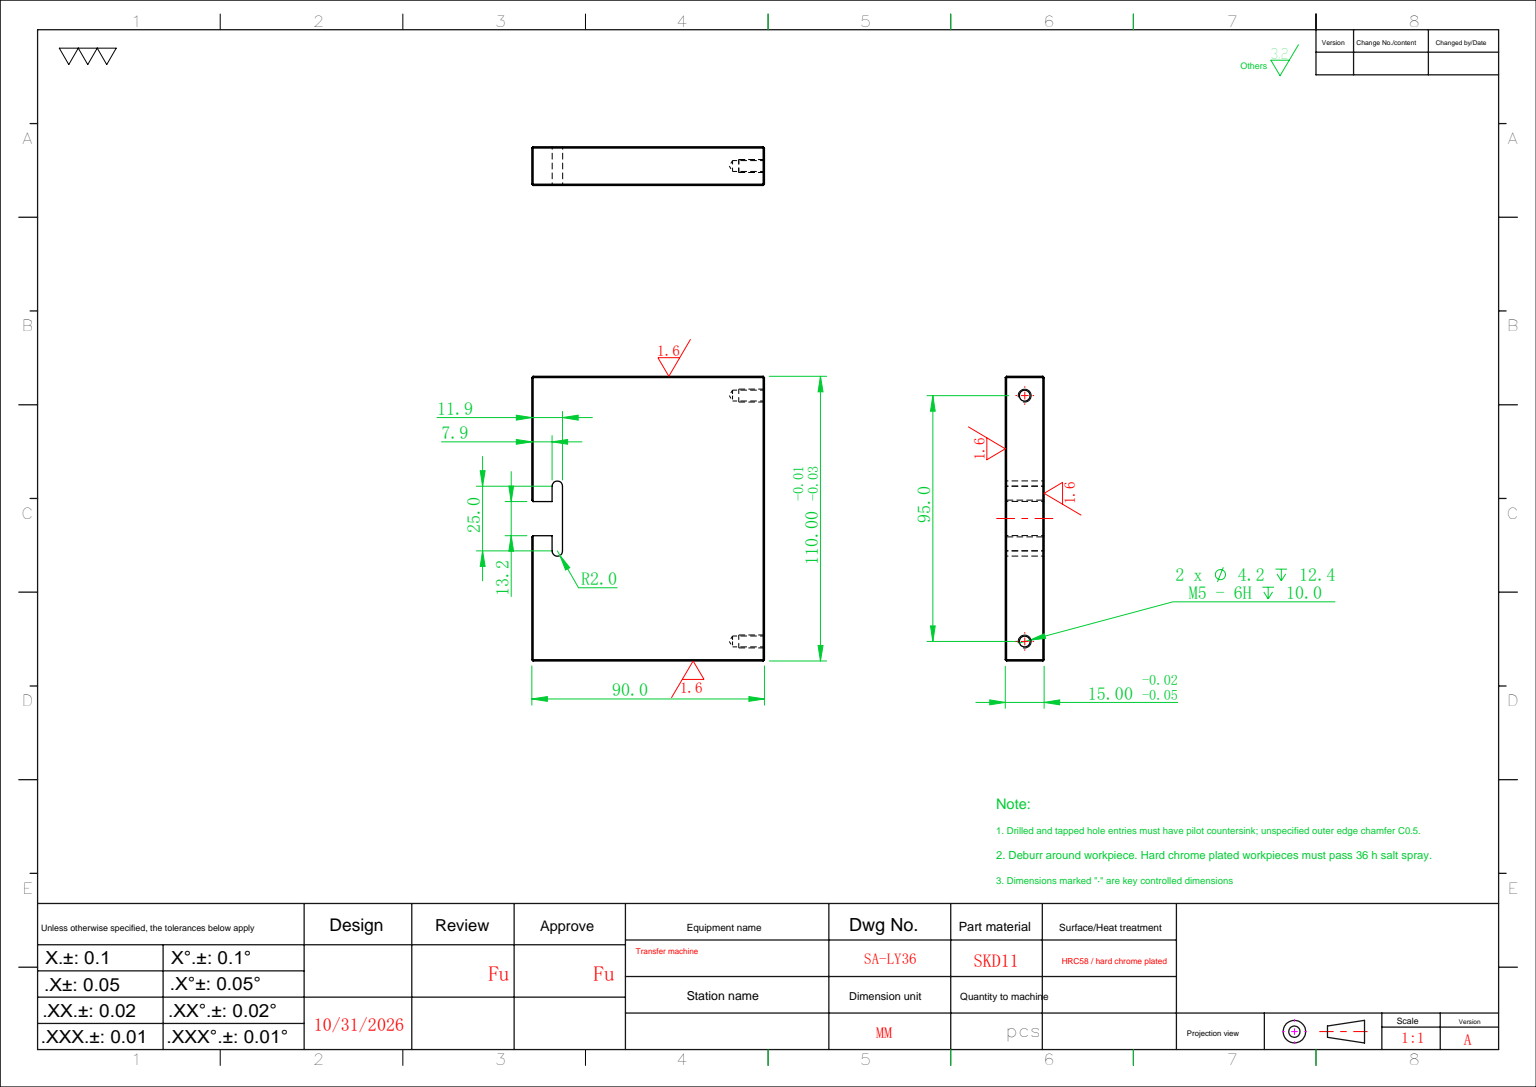
from build123d import *

# Parameters (mm, degrees)
SKETCH_1_W               = 110
SKETCH_1_H               = 90
EXTRUDE_1_DEPTH          = 15
CUT_EXTRUDE_1_DEPTH      = 73.629195232
CUT_EXTRUDE_1_DEPTH_BACK = 73.629195232
SKETCH_2_W               = 13.2
SKETCH_2_H               = 11.9
CUT_EXTRUDE_2_DEPTH      = 73.629195232
HOLE_WIZARD_M5_1_D       = 4.2
HOLE_WIZARD_M5_1_DEPTH   = 12.4
HOLE_WIZARD_M5_1_TIP     = 1.2618073
CHAMFER_1_SIZE           = 0.5


with BuildPart() as part:
    # 草图1 → 凸台-拉伸1 (new body)
    with BuildSketch(Plane.XY):
        Rectangle(SKETCH_1_W, SKETCH_1_H)
    extrude(amount=EXTRUDE_1_DEPTH)

    # 草图2 → 切除-拉伸1 (cut, two sides: drawn at the far end of the back side and taken through both)
    with BuildSketch(Plane.XY.offset(15).offset(-CUT_EXTRUDE_1_DEPTH_BACK)):
        with Locations((0, 39.05)):
            Rectangle(SKETCH_2_W, SKETCH_2_H)
    extrude(amount=CUT_EXTRUDE_1_DEPTH + CUT_EXTRUDE_1_DEPTH_BACK, mode=Mode.SUBTRACT)

    # 草图3 → 切除-拉伸2 (cut, through all)
    with BuildSketch(Plane.XY.offset(15)):
        with BuildLine():
            Line((-12.5, 37.15), (12.5, 37.15))
            ThreePointArc((12.5, 37.15), (14.525, 35.125), (12.5, 33.1))
            Line((12.5, 33.1), (-12.5, 33.1))
            ThreePointArc((-12.5, 33.1), (-14.525, 35.125), (-12.5, 37.15))
        make_face()
    extrude(amount=-CUT_EXTRUDE_2_DEPTH, mode=Mode.SUBTRACT)

    # M5 螺纹孔1
    with Locations(Plane(origin=(0, -45, 0), x_dir=(-1, 0, 0), z_dir=(0, -1, 0))):
        with Locations((-47.5, -7.5), (47.5, -7.5)):
            Hole(HOLE_WIZARD_M5_1_D / 2, depth=HOLE_WIZARD_M5_1_DEPTH)
            with Locations((0, 0, -(HOLE_WIZARD_M5_1_DEPTH + HOLE_WIZARD_M5_1_TIP / 2))):  # 118° drill point
                Cone(0, HOLE_WIZARD_M5_1_D / 2, HOLE_WIZARD_M5_1_TIP, mode=Mode.SUBTRACT)

    # 倒角1
    chamfer_1_edges = [part.edges().sort_by_distance(p)[0] for p in [
        (-55, 0, 15),
        (-30.8, 45, 0),
        (-30.8, 45, 15),
        (0, -45, 15),
        (-6.6, 45, 7.5),
        (6.6, 45, 7.5),
        (55, 0, 15),
        (0, -45, 0),
        (-55, 0, 0),
        (30.8, 45, 0),
        (55, 0, 0),
        (55, -45, 7.5),
        (-55, -45, 7.5),
        (-55, 45, 7.5),
        (55, 45, 7.5),
        (30.8, 45, 15),
    ]]
    chamfer(chamfer_1_edges, length=CHAMFER_1_SIZE)


solid = part.part
